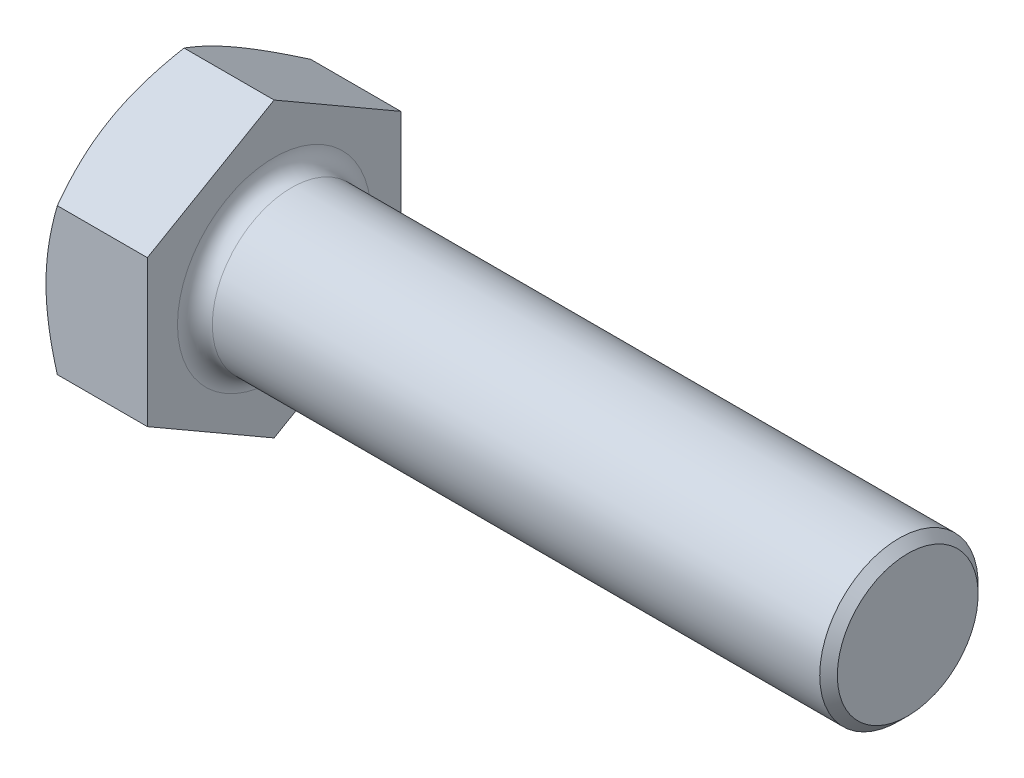
SolidWorks part; units mm, degrees
material "Q235"
ref_plane "Front Plane" through (0, 0, 0) normal (0, 0, 1) x (1, 0, 0)
ref_plane "Top Plane" through (0, 0, 0) normal (0, 1, 0) x (1, 0, 0)
ref_plane "Right Plane" through (0, 0, 0) normal (1, 0, 0) x (0, 0, -1)
sketch "Sketch1" plane through (0, 0, 0) normal (0, 0, 1) x (1, 0, 0)
  line L0 (0, 0) -> (46.4, 0) construction
  line L1 (0, 0) -> (0, 8.795)
  line L2 (0, 8.795) -> (6.4, 8.795)
  line L3 (6.4, 8.795) -> (6.4, 0)
  line L4 (6.4, 5) -> (46.4, 5)
  line L5 (46.4, 5) -> (46.4, 0)
  line L6 (0, 8) -> (0.459, 8.795)
  line L7 (43.4, 5) -> (43.4, 0)
  line L8 (10.9, 5) -> (10.9, 0)
  line L9 (6.4, 4.5129) -> (46.4, 4.5129)
  line L10 (46.4, 4.1881) -> (6.4, 4.1881)
  line L11 (5.8, 7.735) -> (6.4, 7.135)
  line L12 (5.8, 8.795) -> (5.8, 0)
  line L13 (6.3, 7.235) -> (6.3, 0) construction
  arc A0 (6.4, 6.1) -> (7.5, 5) centre (7.5, 6.1) ccw
  point P12 (44.9, 0)
  point P13 (2.23, 8.795)
  point P14 (6.4, 6.1)
  point P24 (6.4, 7.235)
  dimension "D1" = 0.1
  dimension "r" = 1.1
  dimension "k" = 6.4
  dimension "D2" = 45
  dimension "β" = 30
  dimension "e" = 17.59
  dimension "s" = 16
  dimension "d" = 10
  dimension "l" = 40
  dimension "D52" = 3
  dimension "P" = 1.5
  dimension "kw" = 4.17
  dimension "da" = 12.2
  dimension "a" = 4.5
  dimension "ds" = 9.0258
  dimension "D61" = 8.3763
  dimension "dw" = 14.47
  dimension "c" = 0.6
sketch "Sketch2" plane through (0, 0, 0) normal (1, 0, 0) x (0, 0, -1)
  line L1 (0, 9.2376) -> (-8, 4.6188)
  line L2 (-8, 4.6188) -> (-8, -4.6188)
  line L3 (-8, -4.6188) -> (0, -9.2376)
  line L4 (0, -9.2376) -> (8, -4.6188)
  line L5 (8, -4.6188) -> (8, 4.6188)
  line L6 (8, 4.6188) -> (0, 9.2376)
  circle A0 centre (0, 0) radius 8 construction
sketch "Sketch3" plane through (0, 0, 0) normal (1, 0, 0) x (0, 0, -1)
  line L0 (8, 4.6188) -> (0, 9.2376) construction
  line L1 (0, 9.2376) -> (-8, 4.6188) construction
  line L2 (-8, 4.6188) -> (-8, -4.6188) construction
  line L3 (8, -4.6188) -> (8, 4.6188) construction
  line L4 (0, -9.2376) -> (8, -4.6188) construction
  line L5 (-8, -4.6188) -> (0, -9.2376) construction
  line L6 (8, 4.6188) -> (0, 9.2376)
  line L7 (0, 9.2376) -> (-8, 4.6188)
  line L8 (-8, 4.6188) -> (-8, -4.6188)
  line L9 (8, -4.6188) -> (8, 4.6188)
  line L10 (0, -9.2376) -> (8, -4.6188)
  line L11 (-8, -4.6188) -> (0, -9.2376)
extrude "Boss-Extrude1" add sketch "Sketch3" along normal up to vertex (6.4 mm away) up to point (6.4, 8.795, 0)
sketch "Sketch4" plane through (0, 0, 0) normal (-1, 0, 0) x (0, 0, 1)
  circle A0 centre (0, 0) radius 8 construction
  circle A1 centre (0, 0) radius 8
  circle A2 centre (0, 0) radius 17.59
  dimension "D1" = 35.18
extrude "Cut-Extrude1" cut sketch "Sketch4" against normal blind 0.8 draft 60
sketch "Sketch5" plane through (0, 0, 0) normal (0, 0, 1) x (1, 0, 0)
  line L0 (6.4, 5) -> (46.4, 5) construction
  line L1 (46.4, 5) -> (46.4, 0) construction
  line L2 (0, 0) -> (46.4, 0) construction
  line L3 (7.5, 5) -> (46.4, 5)
  line L4 (46.4, 5) -> (46.4, 0)
  line L5 (6.4, 0) -> (46.4, 0)
  line L6 (6.4, 6.1) -> (6.4, 0)
  arc A0 (6.4, 6.1) -> (7.5, 5) centre (7.5, 6.1) ccw construction
  arc A1 (6.4, 6.1) -> (7.5, 5) centre (7.5, 6.1) ccw
revolve "Revolve1" add sketch "Sketch5" angle 360 about L5
cosmetic thread "Cosmetic Thread2" parameters "D1"=35.5, "D2"=8.3763
chamfer "Chamfer2" distance 0.5556 angle 45 1 edges at (46.4, 0, 5)
sketch "Sketch7" plane through (0, 0, 0) normal (0, 0, 1) x (1, 0, 0)
  line L0 (6.4, 7.135) -> (5.8, 7.735)
  line L1 (5.8, 7.735) -> (5.8, 17.59)
  line L2 (5.8, 17.59) -> (6.4, 17.59)
  line L3 (6.4, 17.59) -> (6.4, 7.135)
  line L4 (0, 0) -> (46.4, 0) construction
  line L5 (0, 0) -> (46.4, 0) construction
  dimension "D1" = 35.18
revolve "Cut-Revolve1" [suppressed] cut sketch "Sketch7" angle 360 mid plane about L5
sketch "Sketch6" [suppressed] plane through (0, 0, 0) normal (0, 0, 1) x (1, 0, 0)
  line L0 (5.9, 0) -> (5.9, 2.5) construction
  line L1 (5.9, 2.5) -> (13.5, 2.5)
  line L2 (13.5, 2.5) -> (13.5, 0)
  line L3 (5.9, 2.5) -> (4.069, 2.245)
  line L5 (3.5, 2.2402) -> (13.5, 2.2402) construction
  line L6 (3.5, 4.315) -> (3.5, 0) construction
  line L7 (3.5, 2.7402) -> (3.5, 0)
  line L8 (3.5, 0) -> (13.5, 0)
  arc A0 (4.069, 2.245) -> (3.5, 2.7402) centre (4, 2.7402) cw
  arc A1 (3.5, 3) -> (4, 2.5) centre (4, 3) ccw construction
revolve "Revolve2" add sketch "Sketch6" angle 360 about L8
cosmetic thread "Cosmetic Thread1" [suppressed] parameters "D1"=25.5, "D2"=8.3763
chamfer "Chamfer1" [suppressed] distance 0.5556 angle 45
sketch "Sketch8" plane through (0, 0, 0) normal (0, 0, 1) x (1, 0, 0)
  line L0 (6.4, 7.135) -> (5.8, 7.735)
  line L1 (5.8, 7.735) -> (5.8, 17.59)
  line L2 (5.8, 17.59) -> (6.4, 17.59)
  line L3 (6.4, 17.59) -> (6.4, 7.135)
  line L4 (0, 0) -> (46.4, 0) construction
  line L5 (0, 0) -> (46.4, 0) construction
  dimension "D1" = 35.18
revolve "Cut-Revolve2" [suppressed] cut sketch "Sketch8" angle 360 mid plane about L5
